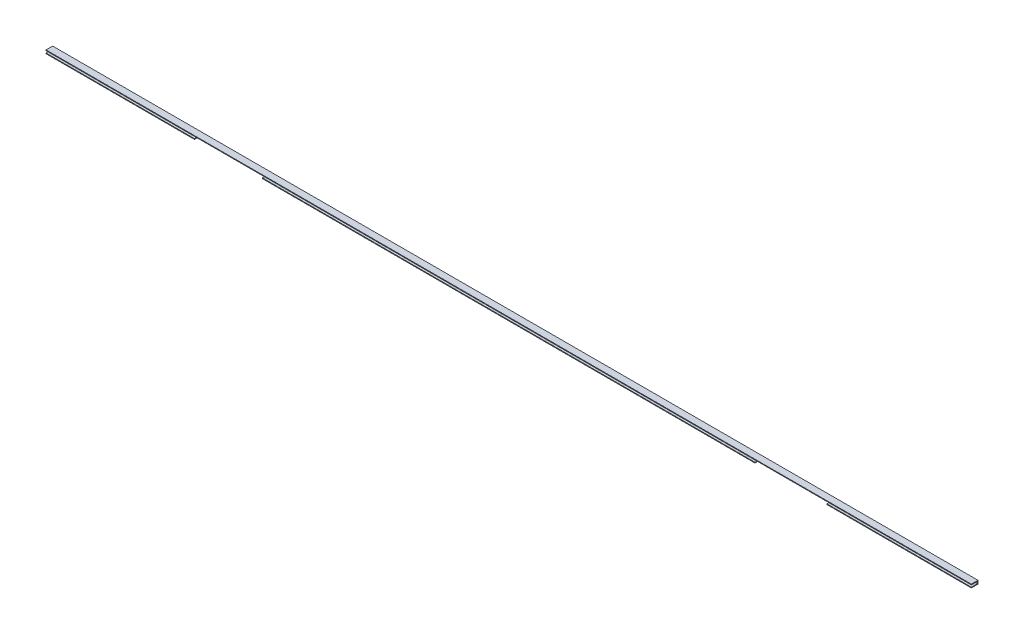
from build123d import *

# Parameters (mm, degrees)
SKETCH_1_W               = 1390
SKETCH_1_H               = 5
SKETCH_1_W_2             = 1388
SKETCH_1_H_2             = 3
EXTRUDE_1_DEPTH          = 10
SKETCH_2_W               = 1
SKETCH_2_H               = 5
EXTRUDE_1_2_DEPTH        = 1389
CUT_EXTRUDE_1_DEPTH      = 1390.038246414
CUT_EXTRUDE_1_DEPTH_BACK = 1390.038246414
SKETCH_3_W               = 9
SKETCH_3_H               = 3
CUT_EXTRUDE_START        = -325
SKETCH_4_W               = 10
SKETCH_4_H               = 1
CUT_EXTRUDE_2_DEPTH      = 102
SKETCH_5_W               = 6
SKETCH_5_H               = 9
CUT_EXTRUDE_5_DEPTH      = 4


with BuildPart() as part:
    # 草图1 → Extrude 1 (new body)
    with BuildSketch(Plane.XY):
        Rectangle(SKETCH_1_W, SKETCH_1_H)
        Rectangle(SKETCH_1_W_2, SKETCH_1_H_2, mode=Mode.SUBTRACT)
    extrude(amount=EXTRUDE_1_DEPTH)

    # 草图2 → Extrude 1 2 (add)
    with BuildSketch(Plane.ZY.offset(695)):
        with Locations((0.5, 0)):
            Rectangle(SKETCH_2_W, SKETCH_2_H)
    extrude(amount=-EXTRUDE_1_2_DEPTH)

    # 草图3 → 切除-拉伸1 (cut, two sides: drawn at the far end of the back side and taken through both)
    with BuildSketch(Plane.ZY.offset(-694).offset(-CUT_EXTRUDE_1_DEPTH_BACK)):
        with Locations((5.5, 0)):
            Rectangle(SKETCH_3_W, SKETCH_3_H)
    extrude(amount=CUT_EXTRUDE_1_DEPTH + CUT_EXTRUDE_1_DEPTH_BACK, mode=Mode.SUBTRACT)

    # 草图4 → 切除-拉伸2 (cut)
    with BuildSketch(Plane.ZY.offset(695).offset(CUT_EXTRUDE_START)):
        with Locations((5, -2)):
            Rectangle(SKETCH_4_W, SKETCH_4_H)
    cut_extrude_2 = extrude(amount=CUT_EXTRUDE_2_DEPTH, mode=Mode.SUBTRACT)

    # 镜向1: 切除-拉伸2 across plane
    add(cut_extrude_2.mirror(Plane(origin=(0, 0, 0), x_dir=(0, 0, 1), z_dir=(1, 0, 0))), mode=Mode.SUBTRACT)

    # 草图5 → 切除-拉伸5 (cut)
    with BuildSketch(Plane.XZ.offset(2.5)):
        with Locations((475, 5.5)):
            Rectangle(SKETCH_5_W, SKETCH_5_H)
    extrude(amount=-CUT_EXTRUDE_5_DEPTH, mode=Mode.SUBTRACT)


solid = part.part
